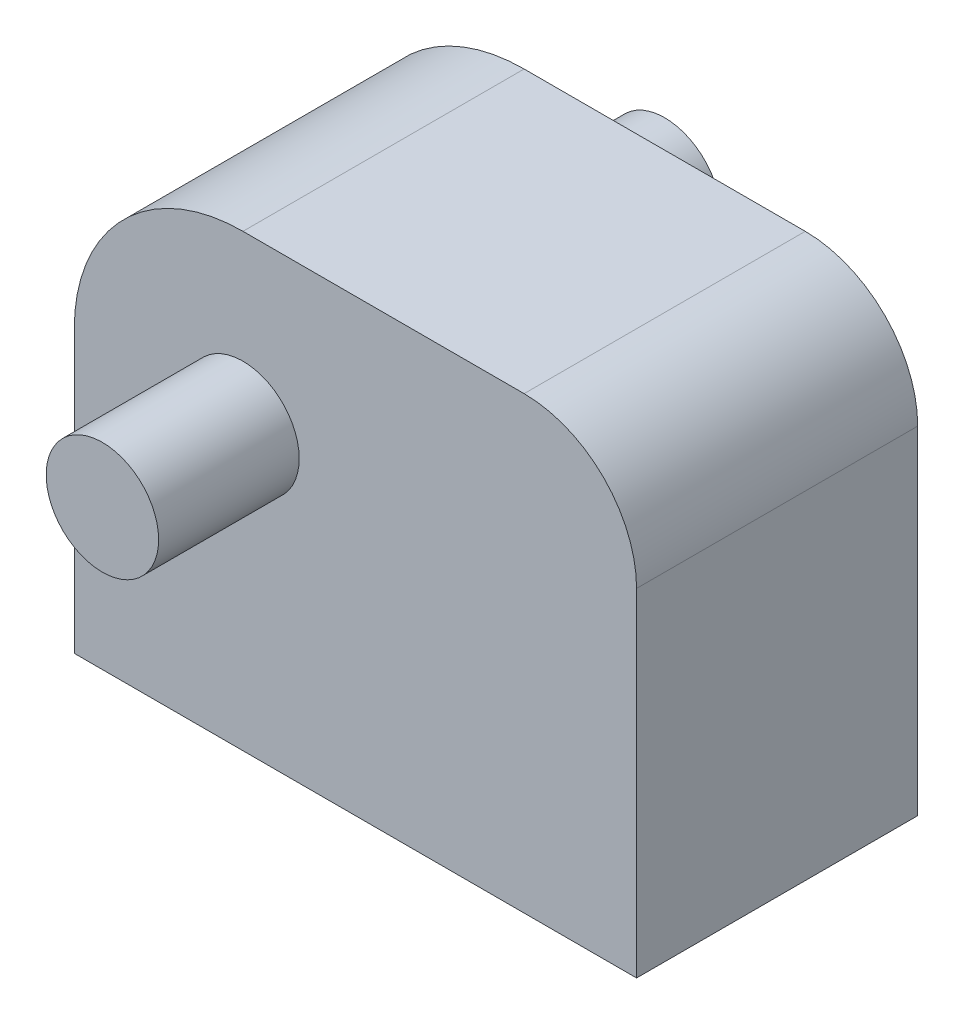
from build123d import *

# Parameters (mm, degrees)
BOSS_EXTRUDE1_DEPTH      = 250
BOSS_EXTRUDE1_DEPTH_BACK = 250
SKETCH1_W                = 1000
SKETCH1_H                = 800
BOSS_EXTRUDE2_DEPTH      = 500
BOSS_EXTRUDE2_DEPTH_BACK = 500
SKETCH2_R                = 100
FILLET1_R                = 300
FILLET2_R                = 200


with BuildPart() as part:
    # Sketch1 → Boss-Extrude1 (new, two sides: drawn at the far end of the back side and taken through both)
    with BuildSketch(Plane.XY.offset(-BOSS_EXTRUDE1_DEPTH_BACK)):
        with Locations((200, -100)):
            Rectangle(SKETCH1_W, SKETCH1_H)
    extrude(amount=BOSS_EXTRUDE1_DEPTH + BOSS_EXTRUDE1_DEPTH_BACK)

    # Sketch2 → Boss-Extrude2 (add, two sides: drawn at the far end of the back side and taken through both)
    with BuildSketch(Plane.XY.offset(-BOSS_EXTRUDE2_DEPTH_BACK)):
        Circle(SKETCH2_R)
    extrude(amount=BOSS_EXTRUDE2_DEPTH + BOSS_EXTRUDE2_DEPTH_BACK)

    # Fillet1
    fillet1_edges = [part.edges().sort_by_distance(p)[0] for p in [
        (-300, 300, 0),
    ]]
    fillet(fillet1_edges, radius=FILLET1_R)

    # Fillet2
    fillet2_edges = [part.edges().sort_by_distance(p)[0] for p in [
        (700, 300, 0),
    ]]
    fillet(fillet2_edges, radius=FILLET2_R)


solid = part.part
